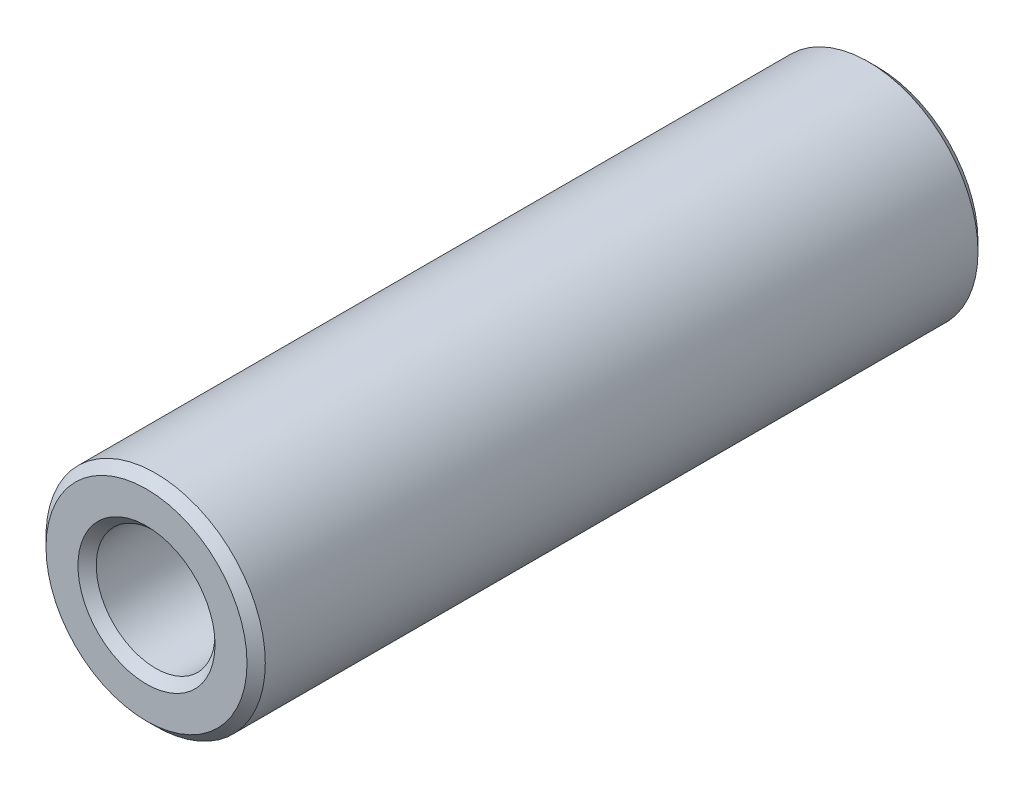
SolidWorks part; units mm, degrees
material "6061-T6"
ref_plane "Front Plane" through (0, 0, 0) normal (0, 0, 1) x (1, 0, 0)
ref_plane "Top Plane" through (0, 0, 0) normal (0, 1, 0) x (1, 0, 0)
ref_plane "Right Plane" through (0, 0, 0) normal (1, 0, 0) x (0, 0, -1)
sketch "Sketch2" plane through (0, 0, 0) normal (0, 1, 0) x (1, 0, 0)
  line L0 (0, 0) -> (0, 4.2658) construction
  line L1 (1.5, 0) -> (2.2, 0)
  line L2 (1.3, 0.2) -> (1.3, 15.8)
  line L3 (1.5, 16) -> (2.2, 16)
  line L4 (2.4, 0.2) -> (2.4, 15.8)
  line L5 (1.3, 0.2) -> (1.5, 0)
  line L6 (2.2, 0) -> (2.4, 0.2)
  line L7 (1.3, 15.8) -> (1.5, 16)
  line L8 (2.2, 16) -> (2.4, 15.8)
  point P0 (1.3, 0)
  point P1 (2.4, 16)
  point P2 (1.3, 16)
  point P3 (2.4, 0)
  dimension "D1" = 2.6
  dimension "D2" = 4.8
  dimension "D3" = 16
revolve "Revolve1" add sketch "Sketch2" angle 360 about L0
